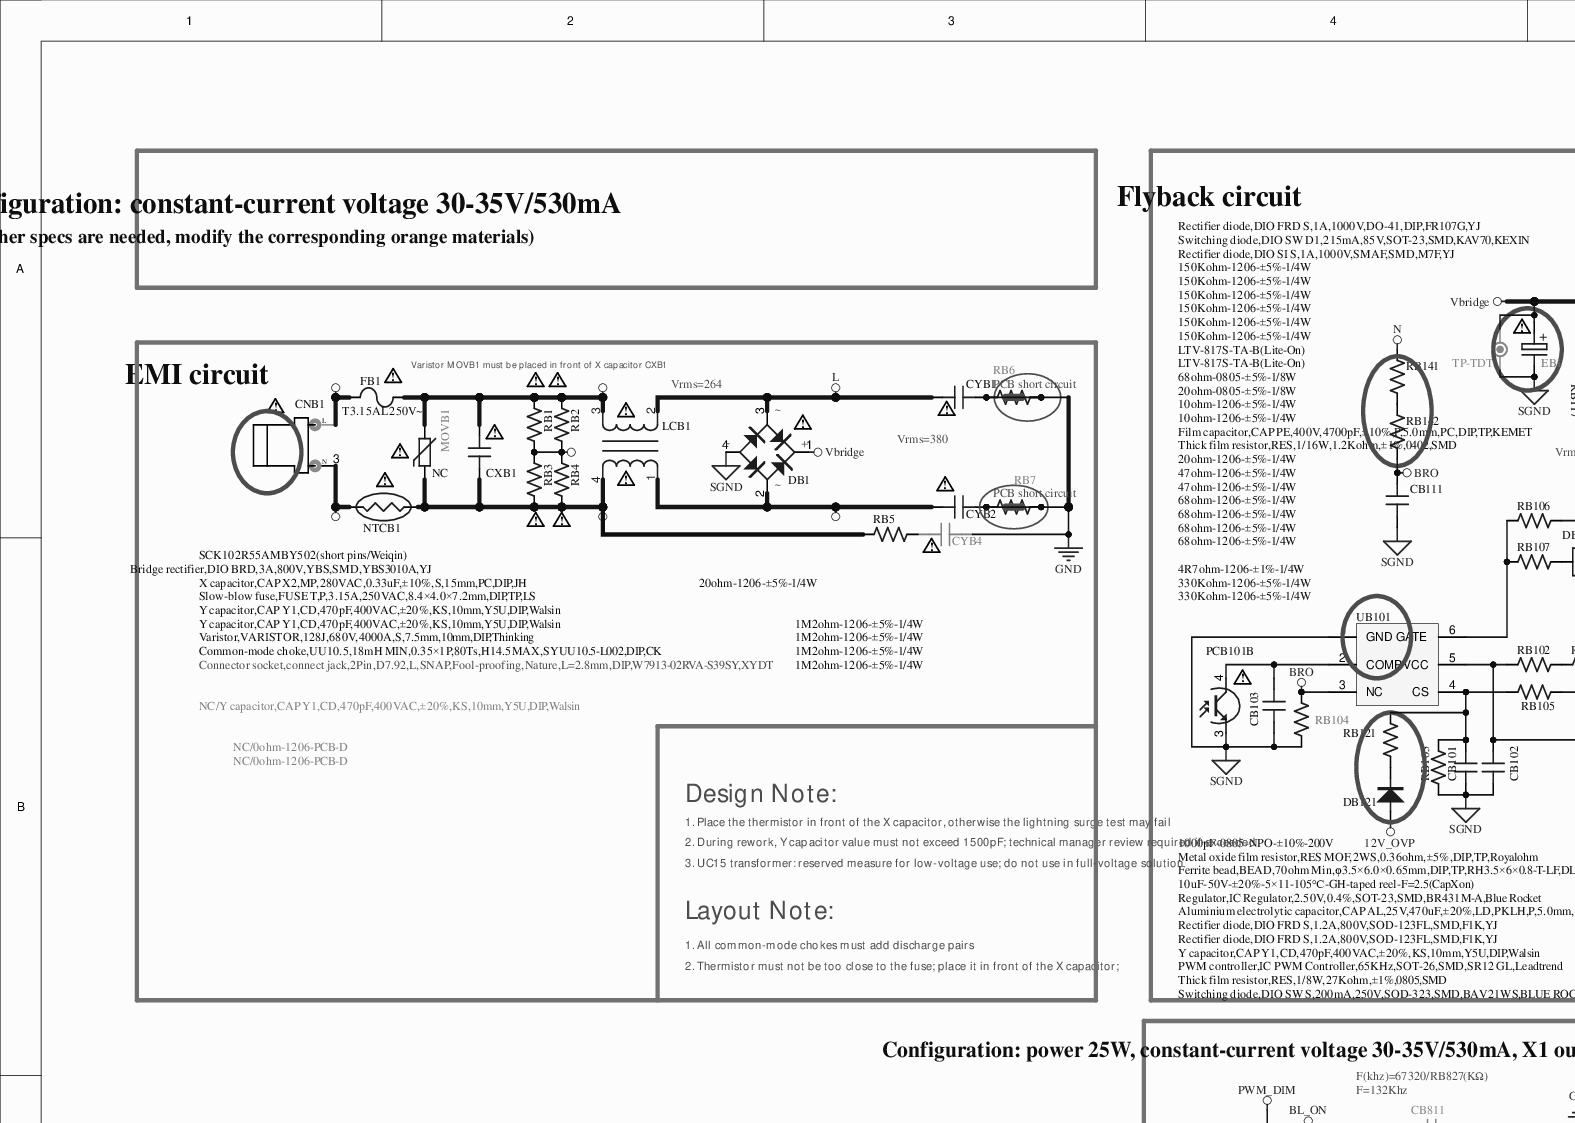
[diagram p0: MISC84395-4.SchDoc, top left]
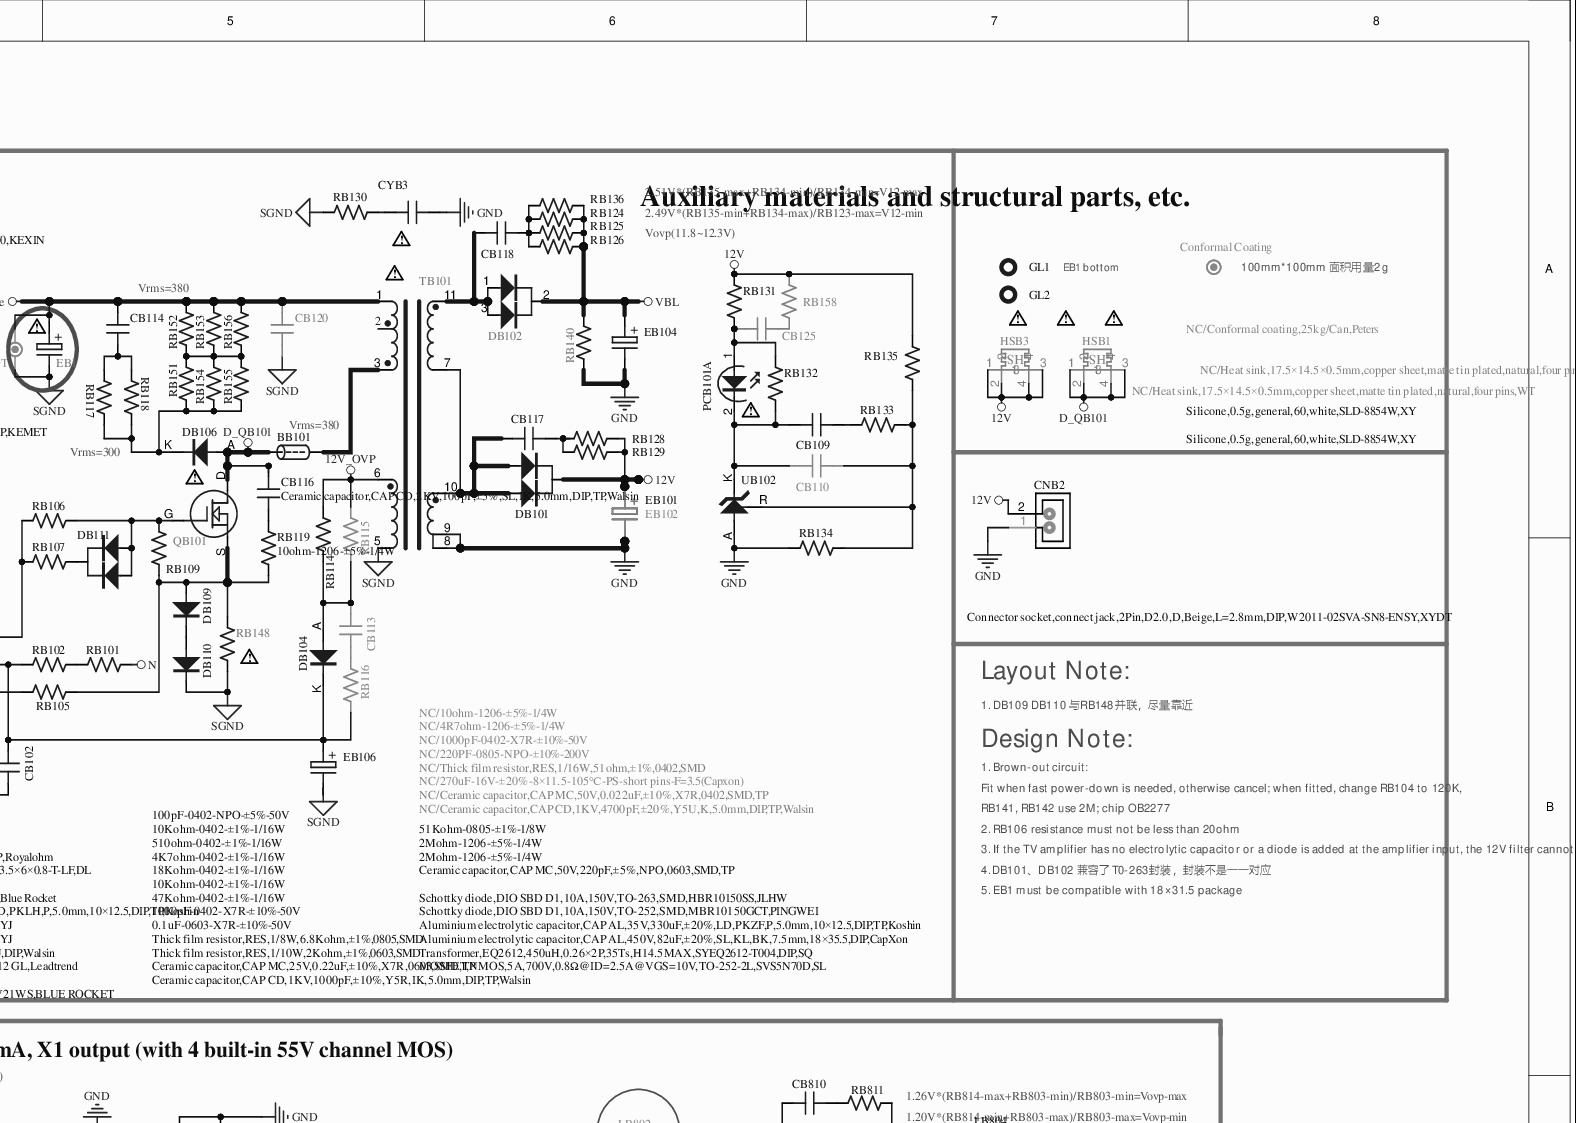
[diagram p1: MISC84395-4.SchDoc, top right]
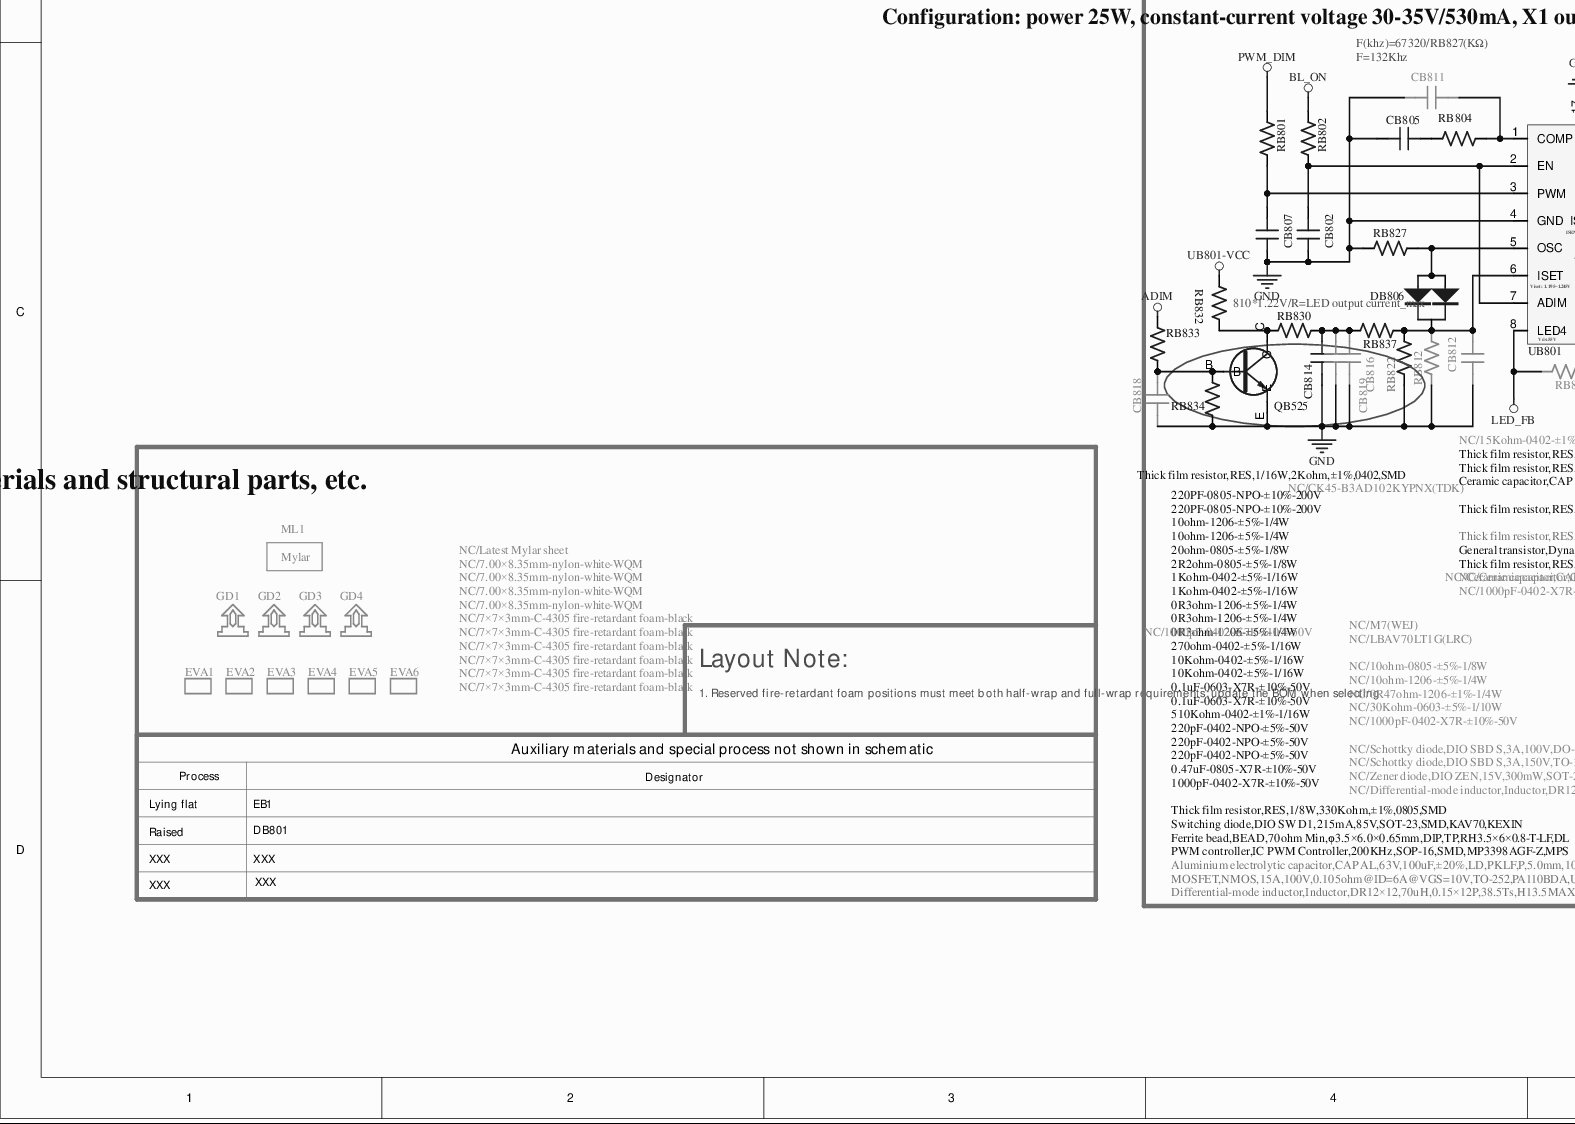
[diagram p2: MISC84395-4.SchDoc, bottom left]
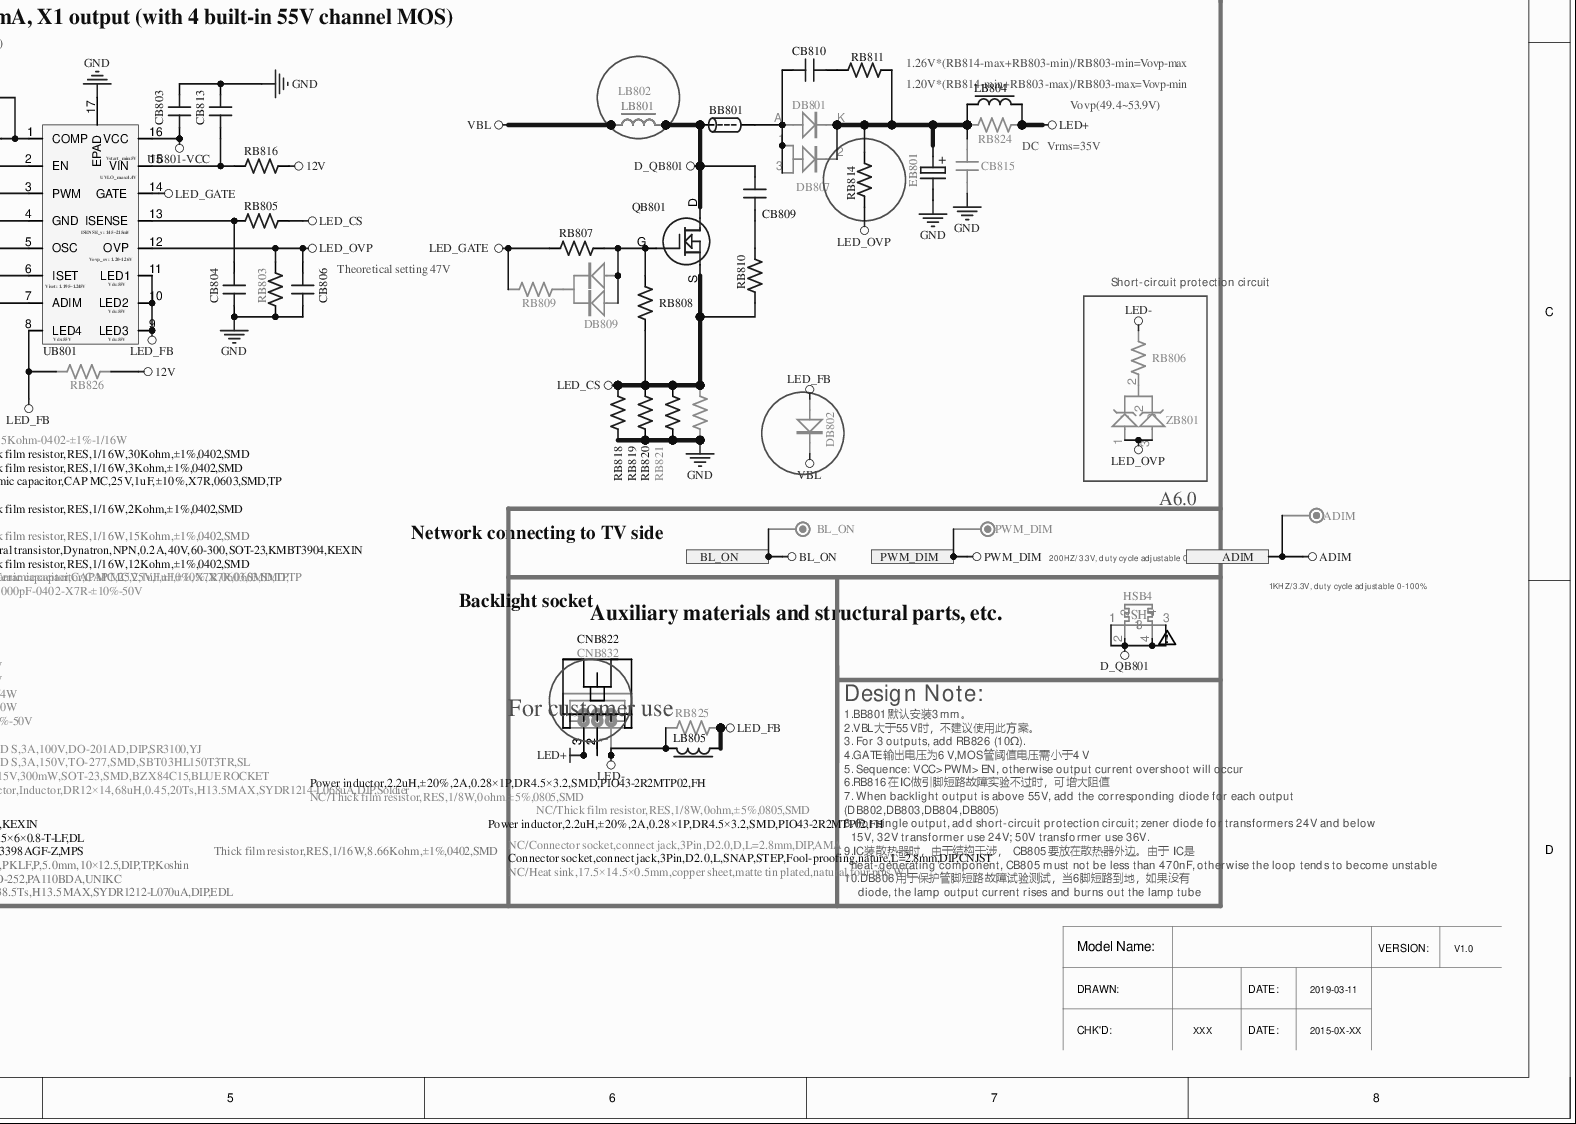
[diagram p3: MISC84395-4.SchDoc, bottom right]
# Altium project MISC84395-37.PrjPCB (part 12 of 13)

## Sheet MISC84395-4.SchDoc: MISC84395
size A2

### Parts
ADIM  NC/TEST  [TP_BL]  (value not drawn)
BB101  Ferrite bead,BEAD,70ohm Min,φ3.5×6.0×0.65mm,DIP,TP,RH3.5×6×0.8-T-LF,DL  [LB/3.5*6*12.5]
BB801  Ferrite bead,BEAD,70ohm Min,φ3.5×6.0×0.65mm,DIP,TP,RH3.5×6×0.8-T-LF,DL  [LB/3.5*6*12.5]
BL_ON  NC/TEST  [TP_BL]  (value not drawn)
CB101  100pF-0402-NPO-±5%-50V  [C0402]
CB102  0.1uF-0603-X7R-±10%-50V  [C0603]
CB103  1000pF-0402-X7R-±10%-50V  [C0402]
CB109  Ceramic capacitor,CAP MC,25V,0.22uF,±10%,X7R,0603,SMD,TP  [C0603]
CB110  NC/1000pF-0402-X7R-±10%-50V  [C0402]
CB111  Ceramic capacitor,CAP MC,50V,220pF,±5%,NPO,0603,SMD,TP  [C0603]
CB113  NC/220PF-0805-NPO-±10%-200V  [C0805]
CB114  Film capacitor,CAP PE,400V,4700pF,±10%,P,5.0mm,PC,DIP,TP,KEMET  [CAP8*2.5-V-5]
CB116  Ceramic capacitor,CAP CD,2KV,100pF,±5%,SL,IK,5.0mm,DIP,TP,Walsin  [CAP6.5*5-V-5-1]
CB117  1000pF-0805-NPO-±10%-200V  [C0805]
CB118  Ceramic capacitor,CAP CD,1KV,1000pF,±10%,Y5R,IK,5.0mm,DIP,TP,Walsin  [CAP8.5*5-V-5]
CB120  NC/Ceramic capacitor,CAP CD,1KV,4700pF,±20%,Y5U,K,5.0mm,DIP,TP,Walsin  [CAP10*4.5-V-5]
CB125  NC/Ceramic capacitor,CAP MC,50V,0.022uF,±10%,X7R,0402,SMD,TP  [C0402]
CB802  220pF-0402-NPO-±5%-50V  [C0402]
CB803  0.1uF-0603-X7R-±10%-50V  [C0603]
CB804  220pF-0402-NPO-±5%-50V  [C0402]
CB805  0.47uF-0805-X7R-±10%-50V  [C0805]
CB806  1000pF-0402-X7R-±10%-50V  [C0402]
CB807  220pF-0402-NPO-±5%-50V  [C0402]
CB809  220PF-0805-NPO-±10%-200V  [C0805]
CB810  220PF-0805-NPO-±10%-200V  [C0805]
CB811  NC/1000pF-0402-X7R-±10%-50V  [C0402]
CB812  NC/1000pF-0402-X7R-±10%-50V  [C0402]
CB813  0.1uF-0603-X7R-±10%-50V  [C0603]
CB814  Ceramic capacitor,CAP MC,25V,1uF,±10%,X7R,0603,SMD,TP  [C0603]
CB815  NC/CK45-B3AD102KYPNX(TDK)  [CAP7.5*2.5-V-5]
CB816  NC/Ceramic capacitor,CAP MC,25V,1uF,±10%,X7R,0603,SMD,TP  [C0603]
CB818  NC/1000pF-0402-X7R-±10%-50V  [C0402]
CB819  NC/Ceramic capacitor,CAP MC,25V,1uF,±10%,X7R,0603,SMD,TP  [C0603]
CNB1  Connector socket,connect jack,2Pin,D7.92,L,SNAP,Fool-proofing,Nature,L=2.8mm,DIP,W7913-02RVA-S39SY,XYDT  [CON2-H7.92]
CNB2  Connector socket,connect jack,2Pin,D2.0,D,Beige,L=2.8mm,DIP,W2011-02SVA-SN8-ENSY,XYDT  [SIP2/2.0D-1]
CNB822  Connector socket,connect jack,3Pin,D2.0,L,SNAP,STEP,Fool-proofing,nature,L=2.8mm,DIP,CNJST  [SIP3H/2.0D-3]
CNB832  NC/Connector socket,connect jack,3Pin,D2.0,D,L=2.8mm,DIP,AMA  [SIP3/2.0D-CP]
Conformal_Coating  NC/Conformal coating,25kg/Can,Peters  [Conformal Coating]
CXB1  X capacitor,CAP X2,MP,280VAC,0.33uF,±10%,S,15mm,PC,DIP,JH  [CAP18*8.5-V-15]
CYB1  Y capacitor,CAP Y1,CD,470pF,400VAC,±20%,KS,10mm,Y5U,DIP,Walsin  [CAP13*5-V-10-1]
CYB2  Y capacitor,CAP Y1,CD,470pF,400VAC,±20%,KS,10mm,Y5U,DIP,Walsin  [CAP13*5-V-10-1]
CYB3  Y capacitor,CAP Y1,CD,470pF,400VAC,±20%,KS,10mm,Y5U,DIP,Walsin  [CAP13*5-V-10-1]
CYB4  NC/Y capacitor,CAP Y1,CD,470pF,400VAC,±20%,KS,10mm,Y5U,DIP,Walsin  [CAP13*5-V-10-1]
DB1  Bridge rectifier,DIO BRD,3A,800V,YBS,SMD,YBS3010A,YJ  [B/YBS3010A]
DB101  Schottky diode,DIO SBD D1,10A,150V,TO-252,SMD,MBR10150GCT,PINGWEI  [D2PAK3]
DB102  Schottky diode,DIO SBD D1,10A,150V,TO-263,SMD,HBR10150SS,JLHW  [D2PAK3]
DB104  Rectifier diode,DIO SI S,1A,1000V,SMAF,SMD,M7F,YJ  [DIODE-S-2]
DB106  Rectifier diode,DIO FRD S,1A,1000V,DO-41,DIP,FR107G,YJ  [D1-H-17.5]
DB109  Rectifier diode,DIO FRD S,1.2A,800V,SOD-123FL,SMD,F1K,YJ  [DIODE-S-14]
DB110  Rectifier diode,DIO FRD S,1.2A,800V,SOD-123FL,SMD,F1K,YJ  [DIODE-S-14]
DB111  Switching diode,DIO SW D1,215mA,85V,SOT-23,SMD,KAV70,KEXIN  [SO-23]
DB121  Switching diode,DIO SW S,200mA,250V,SOD-323,SMD,BAV21WS,BLUE ROCKET  [DIODE-S-12]
DB801  NC/Schottky diode,DIO SBD S,3A,100V,DO-201AD,DIP,SR3100,YJ  [D3-H-20]
DB802  NC/M7(WEJ)  [DIODE-S-2]
DB806  Switching diode,DIO SW D1,215mA,85V,SOT-23,SMD,KAV70,KEXIN  [SO-23]
DB807  NC/Schottky diode,DIO SBD S,3A,150V,TO-277,SMD,SBT03HL150T3TR,SL  [DIODE-S-13]
DB809  NC/LBAV70LT1G(LRC)  [SO-23]
EB1  Aluminium electrolytic capacitor,CAP AL,450V,82uF,±20%,SL,KL,BK,7.5mm,18×35.5,DIP,CapXon  [EC(18*41)-H-7.5-1]
EB101  Aluminium electrolytic capacitor,CAP AL,25V,470uF,±20%,LD,PKLH,P,5.0mm,10×12.5,DIP,TP,Koshin  [EC(10*12.5)-V-5]
EB102  NC/270uF-16V-±20%-8×11.5-105℃-PS-short pins-F=3.5(Capxon)  [EC(8*11)-V-3.5]
EB104  Aluminium electrolytic capacitor,CAP AL,35V,330uF,±20%,LD,PKZF,P,5.0mm,10×12.5,DIP,TP,Koshin  [EC(10*12.5)-V-5]
EB106  10uF-50V-±20%-5×11-105℃-GH-taped reel-F=2.5(CapXon)  [EC(5*11)-V-2.5]
EB801  Aluminium electrolytic capacitor,CAP AL,63V,100uF,±20%,LD,PKLF,P,5.0mm,10×12.5,DIP,TP,Koshin  [EC(10*12.5)-V-5]
EVA1  NC/7×7×3mm-C-4305 fire-retardant foam-black  [EVA(7*7*3)]
EVA2  NC/7×7×3mm-C-4305 fire-retardant foam-black  [EVA(7*7*3)]
EVA3  NC/7×7×3mm-C-4305 fire-retardant foam-black  [EVA(7*7*3)]
EVA4  NC/7×7×3mm-C-4305 fire-retardant foam-black  [EVA(7*7*3)]
EVA5  NC/7×7×3mm-C-4305 fire-retardant foam-black  [EVA(7*7*3)]
EVA6  NC/7×7×3mm-C-4305 fire-retardant foam-black  [EVA(7*7*3)]
FB1  Slow-blow fuse,FUSE T,P,3.15A,250VAC,8.4×4.0×7.2mm,DIP,TP,LS  [FUSE8.5*4-V-5(T3.15AL 250V~)]
GD1  NC/7.00×8.35mm-nylon-white-WQM  [Fixed]
GD2  NC/7.00×8.35mm-nylon-white-WQM  [Fixed]
GD3  NC/7.00×8.35mm-nylon-white-WQM  [Fixed]
GD4  NC/7.00×8.35mm-nylon-white-WQM  [Fixed]
GL1  Silicone,0.5g,general,60,white,SLD-8854W,XY  [Silica gel-15]
GL2  Silicone,0.5g,general,60,white,SLD-8854W,XY  [Silica gel-10]
HSB1  NC/Heat sink,17.5×14.5×0.5mm,copper sheet,matte tin plated,natural,four pins,WT  [HS149-YZ]
HSB3  NC/Heat sink,17.5×14.5×0.5mm,copper sheet,matte tin plated,natural,four pins,WT  [HS149-YZ]
HSB4  NC/Heat sink,17.5×14.5×0.5mm,copper sheet,matte tin plated,natural,four pins,WT  [HS149-YZ]
LB801  Differential-mode inductor,Inductor,DR12×12,70uH,0.15×12P,38.5Ts,H13.5MAX,SYDR1212-L070uA,DIP,EDL  [L/LC2/15*14.5-V7.5]
LB802  NC/Differential-mode inductor,Inductor,DR12×14,68uH,0.45,20Ts,H13.5MAX,SYDR1214-L068uA,DIP,Soldier  [L(13.5*15.5)-V-5]
LB804  Power inductor,2.2uH,±20%,2A,0.28×1P,DR4.5×3.2,SMD,PIO43-2R2MTP02,FH  [L(4.5*3.5)-S]
LB805  Power inductor,2.2uH,±20%,2A,0.28×1P,DR4.5×3.2,SMD,PIO43-2R2MTP02,FH  [L(4.5*3.5)-S]
LCB1  Common-mode choke,UU10.5,18mH MIN,0.35×1P,80Ts,H14.5MAX,SYUU10.5-L002,DIP,CK  [L/UU10.5/10*13-2]
ML1  NC/Latest Mylar sheet  [Mylar]
MOVB1  Varistor,VARISTOR,128J,680V,4000A,S,7.5mm,10mm,DIP,Thinking  [VR(13*5)-V-7.5]
NTCB1  SCK102R55AMBY502(short pins/Weiqin)  [NTC(10*5)-V5]
PCB101  LTV-817S-TA-B(Lite-On)  [OC4-S-1]  (parts A,B of 2)
PWM_DIM  NC/TEST  [TP_BL]  (value not drawn)
QB101  MOSFET,NMOS,5A,700V,0.8Ω@ID=2.5A@VGS=10V,TO-252-2L,SVS5N70D,SL  [TO-252-GDS]
QB525  General transistor,Dynatron,NPN,0.2A,40V,60-300,SOT-23,KMBT3904,KEXIN  [SOT-23]
QB801  MOSFET,NMOS,15A,100V,0.105ohm@ID=6A@VGS=10V,TO-252,PA110BDA,UNIKC  [TO-252-GDS]
RB1  1M2ohm-1206-±5%-1/4W  [R1206]
RB2  1M2ohm-1206-±5%-1/4W  [R1206]
RB3  1M2ohm-1206-±5%-1/4W  [R1206]
RB4  1M2ohm-1206-±5%-1/4W  [R1206]
RB5  20ohm-1206-±5%-1/4W  [R1206]
RB6  NC/0ohm-1206-PCB-D  [R1206SC]
RB7  NC/0ohm-1206-PCB-D  [R1206SC]
RB101  330Kohm-1206-±5%-1/4W  [R1206]
RB102  330Kohm-1206-±5%-1/4W  [R1206]
RB103  Thick film resistor,RES,1/8W,6.8Kohm,±1%,0805,SMD  [R0402]
RB104  47Kohm-0402-±1%-1/16W  [R0402]
RB105  510ohm-0402-±1%-1/16W  [R0402]
RB106  68ohm-0805-±5%-1/8W  [R0805]
RB107  20ohm-0805-±5%-1/8W  [R0805]
RB109  10Kohm-0402-±1%-1/16W  [R0402]
RB114  4R7ohm-1206-±1%-1/4W  [R1206]
RB115  NC/4R7ohm-1206-±5%-1/4W  [R1206]
RB116  NC/10ohm-1206-±5%-1/4W  [R1206]
RB117  10ohm-1206-±5%-1/4W  [R1206]
RB118  10ohm-1206-±5%-1/4W  [R1206]
RB119  10ohm-1206-±5%-1/4W  [R1206]
RB121  Thick film resistor,RES,1/8W,27Kohm,±1%,0805,SMD  [R0805]
RB124  68ohm-1206-±5%-1/4W  [R1206]
RB125  68ohm-1206-±5%-1/4W  [R1206]
RB126  68ohm-1206-±5%-1/4W  [R1206]
RB128  47ohm-1206-±5%-1/4W  [R1206]
RB129  47ohm-1206-±5%-1/4W  [R1206]
RB130  20ohm-1206-±5%-1/4W  [R1206]
RB131  Thick film resistor,RES,1/10W,2Kohm,±1%,0603,SMD  [R0603]
RB132  Thick film resistor,RES,1/16W,1.2Kohm,±1%,0402,SMD  [R0402]
RB133  10Kohm-0402-±1%-1/16W  [R0402]
RB134  4K7ohm-0402-±1%-1/16W  [R0402]
RB135  18Kohm-0402-±1%-1/16W  [R0402]
RB136  68ohm-1206-±5%-1/4W  [R1206]
RB140  51Kohm-0805-±1%-1/8W  [R0805]
RB141  2Mohm-1206-±5%-1/4W  [R1206]
RB142  2Mohm-1206-±5%-1/4W  [R1206]
RB148  Metal oxide film resistor,RES MOF,2WS,0.36ohm,±5%,DIP,TP,Royalohm  [R2-H-17.5]
RB151  150Kohm-1206-±5%-1/4W  [R1206]
RB152  150Kohm-1206-±5%-1/4W  [R1206]
RB153  150Kohm-1206-±5%-1/4W  [R1206]
RB154  150Kohm-1206-±5%-1/4W  [R1206]
RB155  150Kohm-1206-±5%-1/4W  [R1206]
RB156  150Kohm-1206-±5%-1/4W  [R1206]
RB158  NC/Thick film resistor,RES,1/16W,51ohm,±1%,0402,SMD  [R0402]
RB801  1Kohm-0402-±5%-1/16W  [R0402]
RB802  10Kohm-0402-±5%-1/16W  [R0402]
RB803  Thick film resistor,RES,1/16W,8.66Kohm,±1%,0402,SMD  [R0402]
RB804  270ohm-0402-±5%-1/16W  [R0402]
RB805  1Kohm-0402-±5%-1/16W  [R0402]
RB806  NC/30Kohm-0603-±5%-1/10W  [R0603]
RB807  20ohm-0805-±5%-1/8W  [R0805]
RB808  10Kohm-0402-±5%-1/16W  [R0402]
RB809  NC/10ohm-0805-±5%-1/8W  [R0805]
RB810  10ohm-1206-±5%-1/4W  [R1206]
RB811  10ohm-1206-±5%-1/4W  [R1206]
RB812  NC/15Kohm-0402-±1%-1/16W  [R0402]
RB814  Thick film resistor,RES,1/8W,330Kohm,±1%,0805,SMD  [R0805]
RB816  2R2ohm-0805-±5%-1/8W  [R0805]
RB818  0R3ohm-1206-±5%-1/4W  [R1206]
RB819  0R3ohm-1206-±5%-1/4W  [R1206]
RB820  0R3ohm-1206-±5%-1/4W  [R1206]
RB821  NC/0R47ohm-1206-±1%-1/4W  [R1206]
RB822  Thick film resistor,RES,1/16W,15Kohm,±1%,0402,SMD  [R0402]
RB824  NC/Thick film resistor,RES,1/8W,0ohm,±5%,0805,SMD  [R0805]
RB825  NC/Thick film resistor,RES,1/8W,0ohm,±5%,0805,SMD  [R0805]
RB826  NC/10ohm-1206-±5%-1/4W  [R1206]
RB827  510Kohm-0402-±1%-1/16W  [R0402]
RB830  Thick film resistor,RES,1/16W,3Kohm,±1%,0402,SMD  [R0402]
RB832  Thick film resistor,RES,1/16W,30Kohm,±1%,0402,SMD  [R0402]
RB833  Thick film resistor,RES,1/16W,2Kohm,±1%,0402,SMD  [R0402]
RB834  Thick film resistor,RES,1/16W,2Kohm,±1%,0402,SMD  [R0402]
RB837  Thick film resistor,RES,1/16W,12Kohm,±1%,0402,SMD  [R0402]
TB101  Transformer,EQ2612,450uH,0.26×2P,35Ts,H14.5MAX,SYEQ2612-T004,DIP,SQ  [T/EQ2512*11]
TP-TDT  NC/  [TP-TDT]  (value not drawn)
UB101  PWM controller,IC PWM Controller,65KHz,SOT-26,SMD,SR12 GL,Leadtrend  [SOT-26]
UB102  Regulator,IC Regulator,2.50V,0.4%,SOT-23,SMD,BR431M-A,Blue Rocket  [SOT-23-RAK]
UB801  PWM controller,IC PWM Controller,200KHz,SOP-16,SMD,MP3398AGF-Z,MPS  [TSSOP16/0.65-3]
ZB801  NC/Zener diode,DIO ZEN,15V,300mW,SOT-23,SMD,BZX84C15,BLUE ROCKET  [SO-23]

### Blocks framed on the sheet
Short-circuit protection circuit: RB806 ZB801

### Ports
ADIM, BL_ON, PWM_DIM

### Nets
12V: CNB2.2 DB101.2 EB101.1 EB102.1 HSB3.1 HSB3.2 HSB3.3 HSB3.4 RB128.2 RB129.2 RB131.2 RB135.1 RB158.2 RB816.2 RB826.2
12V_OVP: DB121.A RB114.2 RB115.2 TB101.6
ADIM: ADIM.1 RB833.2 ; port ADIM
BL_ON: BL_ON.1 RB802.1 ; port BL_ON
BRO: CB111.2 RB104.2 RB142.1 UB101.3(NC)
D_QB101: BB101.1 CB116.2 DB106.A HSB1.1 HSB1.2 HSB1.3 HSB1.4 QB101.D
D_QB801: BB801.1 CB809.2 HSB4.1 HSB4.2 HSB4.3 HSB4.4 LB801.2 LB802.2 QB801.D
GND: CB802.1 CB803.1 CB804.1 CB805.1 CB806.1 CB807.2 CB811.2 CB812.1 CB813.1 CB814.2 CB815.2 CB816.2 CB818.1 CB819.2 CNB2.1 CYB1.2 CYB2.2 CYB3.2 CYB4.2 EB101.2 EB102.2 EB104.2 EB801.2 QB525.E RB6.1 RB6.2 RB6.3 RB7.1 RB7.2 RB7.3 RB134.1 RB140.2 RB803.1 RB812.1 RB818.2 RB819.2 RB820.2 RB821.2 RB822.1 RB827.1 RB834.1 TB101.8 TB101.9 UB102.A UB801.4(GND) UB801.17(EPAD)
L: CYB1.1 DB1.3 LCB1.2
L-1: CNB1.1 FB1.1
L-2: CXB1.1 FB1.2 LCB1.3 MOVB1.1 RB1.1 RB2.1
L-N: RB1.2 RB2.2 RB3.1 RB4.1
LED+: CNB822.3 CNB832.3 LB804.2 RB824.2
LED-: CNB822.1 CNB832.1 LB805.1 RB806.1 RB825.2
LED_CS: QB801.S RB805.1 RB808.2 RB810.2 RB818.1 RB819.1 RB820.1 RB821.1
LED_FB: DB802.A LB805.2 RB825.1 RB826.1 UB801.8(LED4) UB801.9(LED3) UB801.10(LED2) UB801.11(LED1)
LED_GATE: RB807.1 RB809.1 UB801.14(GATE)
LED_OVP: CB806.2 RB803.2 RB814.1 UB801.12(OVP) ZB801.1 ZB801.3
N: CYB2.1 DB1.2 LCB1.1 RB101.1 RB141.2
N-1: CNB1.3 NTCB1.2
N-2: CXB1.2 LCB1.4 MOVB1.2 NTCB1.1 RB3.2 RB4.2 RB5.2
PWM_DIM: PWM_DIM.1 RB801.1 ; port PWM_DIM
SGND: CB101.2 CB102.2 CB103.2 CB111.1 CB120.1 DB1.4 DB110.K EB1.2 EB106.2 PCB101.3 RB103.1 RB104.1 RB130.1 RB148.1 TB101.5 TP-TDT.2 UB101.1(GND)
UB801-VCC: CB803.2 RB832.1 UB801.16(VCC)
VBL: DB102.2 DB802.K EB104.1 LB801.1 LB802.1 RB124.2 RB125.2 RB126.2 RB136.2 RB140.1
Vbridge: CB114.2 CB120.2 DB1.1 EB1.1 RB152.2 RB153.2 RB156.2 TB101.1 TP-TDT.1
NetBB101_2: BB101.2 TB101.3
NetBB801_2: BB801.2 CB810.2 DB801.A DB807.1(Anode_1) DB807.3(Anode_2)
NetCB101_1: CB101.1 RB103.2 RB105.1 RB121.2 UB101.4(CS)
NetCB102_1: CB102.1 DB104.K EB106.1 RB102.1 RB116.1 UB101.5(VCC)
NetCB103_1: CB103.1 PCB101.4 UB101.2(COMP)
NetCB109_1: CB109.1 CB110.1 PCB101.2 RB132.1 UB102.K
NetCB109_2: CB109.2 RB133.1
NetCB110_2: CB110.2 RB133.2 RB134.2 RB135.2 UB102.R
NetCB113_1: CB113.1 DB104.A RB114.1 RB115.1
NetCB113_2: CB113.2 RB116.2
NetCB114_1: CB114.1 RB117.1 RB118.1
NetCB116_1: CB116.1 RB119.2
NetCB117_1: CB117.1 DB101.1 DB101.3 TB101.7 TB101.10
NetCB117_2: CB117.2 RB128.1 RB129.1
NetCB118_1: CB118.1 DB102.1 DB102.3 TB101.11
NetCB118_2: CB118.2 RB124.1 RB125.1 RB126.1 RB136.1
NetCB125_1: CB125.1 PCB101.1 RB131.1 RB132.2
NetCB125_2: CB125.2 RB158.1
NetCB802_2: CB802.2 RB802.2 UB801.2(EN) UB801.7(ADIM)
NetCB804_2: CB804.2 RB805.2 UB801.13(ISENSE)
NetCB805_2: CB805.2 RB804.1
NetCB807_1: CB807.1 RB801.2 UB801.3(PWM)
NetCB809_1: CB809.1 RB810.1
NetCB810_1: CB810.1 RB811.1
NetCB811_1: CB811.1 RB804.2 UB801.1(COMP)
NetCB812_2: CB812.2 DB806.2 RB812.2 RB822.2 RB837.2 UB801.6(ISET)
NetCB813_2: CB813.2 RB816.1 UB801.15(VIN)
NetCB814_1: CB814.1 CB816.1 CB819.1 RB830.1 RB837.1
NetCB815_1: CB815.1 DB801.K DB807.2 EB801.1 LB804.1 RB811.2 RB814.2 RB824.1
NetCB818_2: CB818.2 QB525.B RB833.1 RB834.2
NetCNB822_2: CNB822.2 CNB832.2
NetCYB3_1: CYB3.1 RB130.2
NetCYB4_1: CYB4.1 RB5.1
NetDB106_K: DB106.K RB117.2 RB118.2 RB151.1 RB154.1 RB155.1
NetDB109_A: DB109.A QB101.S RB105.2 RB109.1 RB119.1 RB148.2
NetDB109_K: DB109.K DB110.A
NetDB111_1: DB111.1 DB111.3 QB101.G RB106.2 RB109.2
NetDB111_2: DB111.2 RB107.2
NetDB121_K: DB121.K RB121.1
NetDB806_1: DB806.1 DB806.3 RB827.2 UB801.5(OSC)
NetDB809_1: DB809.1 DB809.3 QB801.G RB807.2 RB808.1
NetDB809_2: DB809.2 RB809.2
NetQB525_C: QB525.C RB830.2 RB832.2
NetRB101_2: RB101.2 RB102.2
NetRB106_1: RB106.1 RB107.1 UB101.6(GATE)
NetRB141_1: RB141.1 RB142.2
NetRB151_2: RB151.2 RB152.1 RB153.1 RB154.2 RB155.2 RB156.1
NetRB806_2: RB806.2 ZB801.2

### Layout directives
net class HOT: 12V, 12V_OVP, ADIM, BL_ON, BRO, D_QB101, D_QB801, GND, L, L-1, L-2, L-N, LED+, LED-, LED_CS, LED_FB, LED_GATE, LED_OVP, N, N-1, N-2, PWM_DIM, SGND, UB801-VCC, VBL, Vbridge
net class POWER: 12V, 12V_OVP, ADIM, BL_ON, BRO, D_QB101, D_QB801, GND, L, L-1, L-2, L-N, LED+, LED-, LED_CS, LED_FB, LED_GATE, LED_OVP, N, N-1, N-2, PWM_DIM, SGND, UB801-VCC, VBL, Vbridge

### Notes on the sheet
- (If other specs are needed, modify the corresponding orange materials)
- Configuration: constant-current voltage 30-35V/530mA
- Flyback circuit
- (near CYB3) !
- 2.51V*(RB135-max+RB134-min)/RB134-min=V12-max
- 2.49V*(RB135-min+RB134-max)/RB123-max=V12-min
- Vovp(11.8~12.3V)
- (near RB136) Auxiliary materials and structural parts, etc.
- (near EB1) !
- Vrms=380
- (near TB101) !
- (near GL2) !
- EB1 bottom
- !
- (near HSB1) !
- (near Conformal_Coating) 100mm*100mm面积用量2g
- EMI circuit
- (near FB1) !
- Varistor MOVB1 must be placed in front of X capacitor CXB1
- Vrms=264
- (near CNB1) !
- (near MOVB1) !
- (near CXB1) !
- (near LCB1) !
- (near DB1) !
- (near CYB1) Vrms=380
- (near CYB1) !
- Vrms=300
- (near BB101) Vrms=380
- (near NTCB1) !
- (near MOVB1) NC
- (near RB4) !
- (near CYB2) !
- (near QB101) !
- (near CYB4) !
- (near RB148) !
- 1. DB109 DB110与RB148并联，尽量靠近
- Layout Note:
- Design Note:
- 1. Brown-out circuit:
- Fit when fast power-down is needed, otherwise cancel; when fitted, change RB104 to 120K,
- RB141, RB142 use 2M; chip OB2277
- 1. Place the thermistor in front of the X capacitor, otherwise the lightning surge test may fail
- (near DB121) 2. During rework, Y capacitor value must not exceed 1500pF; technical manager review required if exceeded
- 3. UC15 transformer: reserved measure for low-voltage use; do not use in full-voltage solution
- 3. If the TV amplifier has no electrolytic capacitor or a diode is added at the amplifier input, the 12V filter cannot use solid-state; two aluminium electrolytics are required
- 4. DB101、DB102兼容了T0-263封装，封装不是一一对应
- 2. RB106 resistance must not be less than 20ohm
- 1. All common-mode chokes must add discharge pairs
- 5. EB1 must be compatible with 18×31.5 package
- 2. Thermistor must not be too close to the fuse; place it in front of the X capacitor;
- (near CB811) F(khz)=67320/RB827(KΩ)
- Configuration: power 25W, constant-current voltage 30-35V/530mA, X1 output (with 4 built-in 55V channel MOS)
- (near CB811) F=132Khz
- 1.26V*(RB814-max+RB803-min)/RB803-min=Vovp-max
- (near LB804) 1.20V*(RB814-min+RB803-max)/RB803-max=Vovp-min
- Vovp(49.4~53.9V)
- (near RB824) DC   Vrms=35V
- (near DB806) 810*1.22V/R=LED output current_max
- Theoretical setting 47V
- (near ML1) Auxiliary materials and structural parts, etc.
- A6.0
- Network connecting to TV side
- 200HZ/3.3V, duty cycle adjustable 0-100%
- 1KHZ/3.3V, duty cycle adjustable 0-100%
- Backlight socket
- Auxiliary materials and structural parts, etc.
- (near HSB4) !
- 1. Reserved fire-retardant foam positions must meet both half-wrap and full-wrap requirements; update the BOM when selecting
- For customer use
- 1.BB801默认安装3mm。
- 2.VBL大于55V时，不建议使用此方案。
- Process
- Auxiliary materials and special process not shown in schematic
- Designator
- 6.RB816在IC做引脚短路故障实验不过时，可增大阻值
- 3. For 3 outputs, add RB826 (10Ω).
- 7. When backlight output is above 55V, add the corresponding diode for each output
- 4.GATE输出电压为6V,MOS管阈值电压需小于4V
- 5. Sequence: VCC>PWM>EN, otherwise output current overshoot will occur
- Lying flat
- Raised
- XXX
- EB1
- DB801
- 8. For single output, add short-circuit protection circuit; zener diode for transformers 24V and below
- (DB802,DB803,DB804,DB805)
- 9.IC装散热器时，由于结构干涉，CB805要放在散热器外边。由于IC是
- 15V, 32V transformer use 24V; 50V transformer use 36V.
- heat-generating component, CB805 must not be less than 470nF, otherwise the loop tends to become unstable
- 10.DB806用于保护管脚短路故障试验测试，当6脚短路到地，如果没有
- diode, the lamp output current rises and burns out the lamp tube
- Model Name:
- DRAWN:
- XXXXXXXXXXXXXXX
- PERSON_A
- DATE:
- 2019-03-11
- VERSION:
- V1.0
- CHK'D:
- 2015-0X-XX
- Title
- Size:
- Date:
- A4
- Number:
- Time:
- Revision:
- Sheet
- of
- File:

### Library data of the parts
ADIM BL_ON PWM_DIM TP-TDT = TEST
BB101 = φ3.5×6.0×0.65mm-CP(编带/秀益达)-DAI: Through-hole ferrite bead
BB801 = φ3.5×6.0×0.65mm-CP(编带/秀益达)-DLAI: Through-hole ferrite bead
CB101 = 100pF-0402-NPO-±5%-50V-D
CB102 CB109 CB803 CB813 CB814 CB816 CB819 = 0.1uF-0603-X7R-±10%-50V-D: CAP
CB103 = 1000pF-0402-X7R-±10%-50V-D
CB110 CB125 CB806 CB811 CB812 CB818 = 1000pF-0402-X7R-±10%-50V-D: CAP
CB111 = 陶瓷电容,CAP MC,25V,1uF,±10%,X7R,0603,SMD,TP-D
CB113 CB809 CB810 = 220PF-0805-NPO-±10%-200V-D: CAP
CB114 = C242G472J20A201(编带/法拉)-DAI: CAP
CB116 = 004.003.0001889-DHAI: Ceramic capacitor,CAP CD,1KV,100pF,±5%,SL,OK,5.0mm,DIP,TP,TDK-DHAI
CB117 = 1000pF-0805-NPO-±10%-200V-D: CAP
CB118 = 004.003.0001892-DHAI: Ceramic capacitor,CAP CD,1KV,220pF,±5%,SL,OK,5.0mm,DIP,TP,TDK-DHAI
CB120 = 004.003.0001665: Ceramic capacitor,CAP CD,1KV,4700pF,±20%,Y5U,K,5.0mm,DIP,TP,Walsin-DHAI
CB802 CB804 CB807 = 220pF-0402-NPO-±5%-50V-D
CB805 = 0.47uF-0805-X7R-±10%-50V-D
CB815 = CK45-B3AD102KYPNX(TDK)-DHAI: CAP
CNB1 = 连接插座,connect jack,2Pin,D7.92,L,SNAP,Fool-proofing,nature,L=2.8mm,DIP,AMA-DLMI: AC socket
CNB2 = XXX.XXX.0001753: Connector socket,connect jack,2Pin,D2.0,D,L=2.8mm,DIP,AMA-DHMI
CNB822 = XXX.XXX.0001725-DLMI: Connector socket,connect jack,3Pin,D2.0,L,SNAP,STEP,Nature,L=2.8mm,DIP,AMA-DLMI
CNB832 = XXX.XXX.0001754: Connector socket,connect jack,3Pin,D2.0,D,L=2.8mm,DIP,AMA-DHMI
Conformal_Coating = 三防漆,25kg/Can,Peters
CXB1 = X电容,CAP X2,MP,275VAC,0.47uF,±10%,S,15mm-Mini,PC,DIP,BM-DHMI: CAP
CYB1-CYB4 = Y电容,CAP Y1,CD,470pF,400VAC,±20%,KS,10mm,Y5U,DIP,Walsin-DHMI: Y1 capacitor
DB1 = 004.005.0000860-D: Bridge rectifier,DIO BRD,3A,800V,YBS,SMD,YBS3010A,YJ-D
DB101 = MBRB10150CT(GOOD-ARK)-D: Diode
DB102 = 整流二极管,DIO FRD D1,10A,400V,TO-263,SMD,MURB1040CT,GOOD-ARK-D: Diode
DB104 DB802 = M7(WEJ)-D: Diode
DB106 = FR107(编带/LRC)-DLAI: Diode
DB109 DB110 = 整流二极管,DIO FRD S,1.2A,800V,eSGA,SMD,R12K,GOOD-ARK-D
DB111 DB806 DB809 = LBAV70LT1G(LRC)-D: Diode
DB121 = BAV21WS-D: Diode
DB801 = SR310(编带/台半)-DLMI: Diode
DB807 = TSPB5H150S-D: Diode
EB1 = 100uF-450V-±20%-18×41-105℃-KS-折脚开槽(CapXon)-S对策-DLMI: Electrolytic
EB101 = 470uF-25V-±20%-10×12.5-105℃-GF-编带-F=5.0(CapXon)-DHAI: Electrolytic
EB102 = 270uF-16V-±20%-8×11.5-105℃-PS-短脚-F=3.5(Capxon): Solid-state
EB104 = 330uF-35V-±20%-10×12.5-105℃-GF-编带-F=5.0(Capxon)-DHAI: Electrolytic
EB106 = 10uF-50V-±20%-5×11-105℃-GH-编带-F=2.5(CapXon)-DHAI: Electrolytic
EB801 = 100uF-63V-±20%-10×12.5-105℃-GF-编带-F=5.0(CapXon)-DHAI: Electrolytic
EVA1-EVA6 = 7×7×3mm-C-4305防火泡棉-黑色-DLMI: EVA
FB1 = 004.026.0000010-DHMI: Slow-blow fuse,FUSE T,P,3.15A,250VAC,8.5×4.0×8mm,DIP,TP,Walter-DHMI
GD1-GD4 = 7.00×8.35mm-尼龙-白色-WQM-DHMI: Mylar stud
GL1 GL2 = 005.002.0000011: Silicone,0.2g,general,60,white,SLD-8854W,XY-DHMI
HSB1 HSB3 HSB4 = 004.040.0006600-DHMI: Heat sink,17.5×14.5×0.5mm,copper sheet,matte tin plated,natural,four pins,WT-DHMI
LB801 = SYDR1212-L003-EDL-DHMI: I-core inductor
LB802 = 差模电感,Inductor,DR12×14,68uH,0.45,20Ts,H13.5MAX,SYDR1214-L068uA,DIP,Soldier-DHMI: I-core inductor
LB804 LB805 = 004.004.0001664: Power inductor,2.2uH,±20%,2A,0.28×1P,DR4.5×3.2,SMD,CD43-2.2uH,wenshan-D
LCB1 = SYUU10.5-L002-JM-DHMI: Common mode
ML1 = MALAY
MOVB1 = TVR10561KSW(为勤)-DHMI: Varistor
NTCB1 = SCK102R55AMBY502(短脚/为勤)-DHMI: Thermistor
PCB101 = LTV-817S-TA-B(光宝)-DMI: Optocoupler
QB101 = 场效应管,NMOS,5.2,650V,1.02ohm@ID=2.6A@VGS=10V,DPAK,TK5P65W,TOSHIBA-D: N Channel Single MOSFET
QB525 = LMBT3904LT1G-D-NPN: Q-NPN-#-#-#
QB801 = ME15N10(松木)-D: N Channel Single MOSFET
RB1-RB4 = 1M2ohm-1206-±5%-1/4W-D: RES
RB5 RB101 RB102 = 330Kohm-1206-±5%-1/4W-D: RES
RB6 RB7 = 0ohm-1206-PCB-D
RB103 RB109 RB133 = 10Kohm-0402-±1%-1/16W-D
RB104 = 47Kohm-0402-±1%-1/16W-D
RB105 = 510ohm-0402-±1%-1/16W-D
RB106 RB121 = 68ohm-0805-±5%-1/8W-D
RB107 RB807 RB824 RB825 = 20ohm-0805-±5%-1/8W-D: RES
RB114 = 4R7ohm-1206-±1%-1/4W-D: RES
RB115 = 4R7ohm-1206-±5%-1/4W-D: RES
RB116-RB119 RB810 RB811 RB826 RB830 RB832-RB834 RB837 = 10ohm-1206-±5%-1/4W-D: RES
RB124-RB126 RB136 = 68ohm-1206-±5%-1/4W-D
RB128 RB129 = 47ohm-1206-±5%-1/4W-D: RES
RB130 = 20ohm-1206-±5%-1/4W-D
RB131 = 1Kohm-0603-±1%-1/10W-D
RB132 = 1Kohm-0402-±1%-1/16W-D
RB134 = 4K7ohm-0402-±1%-1/16W-D: RES
RB135 = 18Kohm-0402-±1%-1/16W-D: RES
RB140 = 51Kohm-0805-±1%-1/8W-D: RES
RB141 RB142 = 2Mohm-1206-±5%-1/4W-D: RES
RB148 = MOF-0R27ohm-±5%-2WS(编带/Futaba)-DLAI: RES
RB151-RB156 = 100Kohm-1206-±5%-1/4W-D: RES
RB158 = 3Kohm-0402-±1%-1/16W-D
RB801 = 1Kohm-0402-±5%-1/16W-D
RB802 RB808 = 10Kohm-0402-±5%-1/16W-D: RES
RB803 = 8K06ohm-0402-±1%-1/16W-D
RB804 = 270ohm-0402-±5%-1/16W-D
RB805 = 1Kohm-0402-±5%-1/16W-D: R
RB806 = 30Kohm-0603-±5%-1/10W-D
RB809 = 10ohm-0805-±5%-1/8W-D
RB812 = 18Kohm-0402-±1%-1/16W-D
RB814 = 004.002.0001276: Thick film resistor,RES,1/8W,330Kohm,±1%,0805-Auto,SMD-D
RB816 = 2R2ohm-0805-±5%-1/8W-D
RB818-RB821 = 0R68ohm-1206-±5%-1/4W-D
RB822 = 15Kohm-0402-±1%-1/16W-D
RB827 = 560kohm-0402-±1%-1/16W-D
TB101 = SYEQ2612-T002-JM-DLMI: Transformer
UB101 = 004.010.0000426: PWM controller,IC PWM Controller,65KHZ,SOT23-6,SMD,OB2273C,ON-Bright-D
UB102 = AZ431AN-ATRE1(BCD)-D: SMD 431
UB801 = MP3398AGF-Z(MPS)-D: IC
ZB801 = BZX84C24(蓝箭)-D: Diode